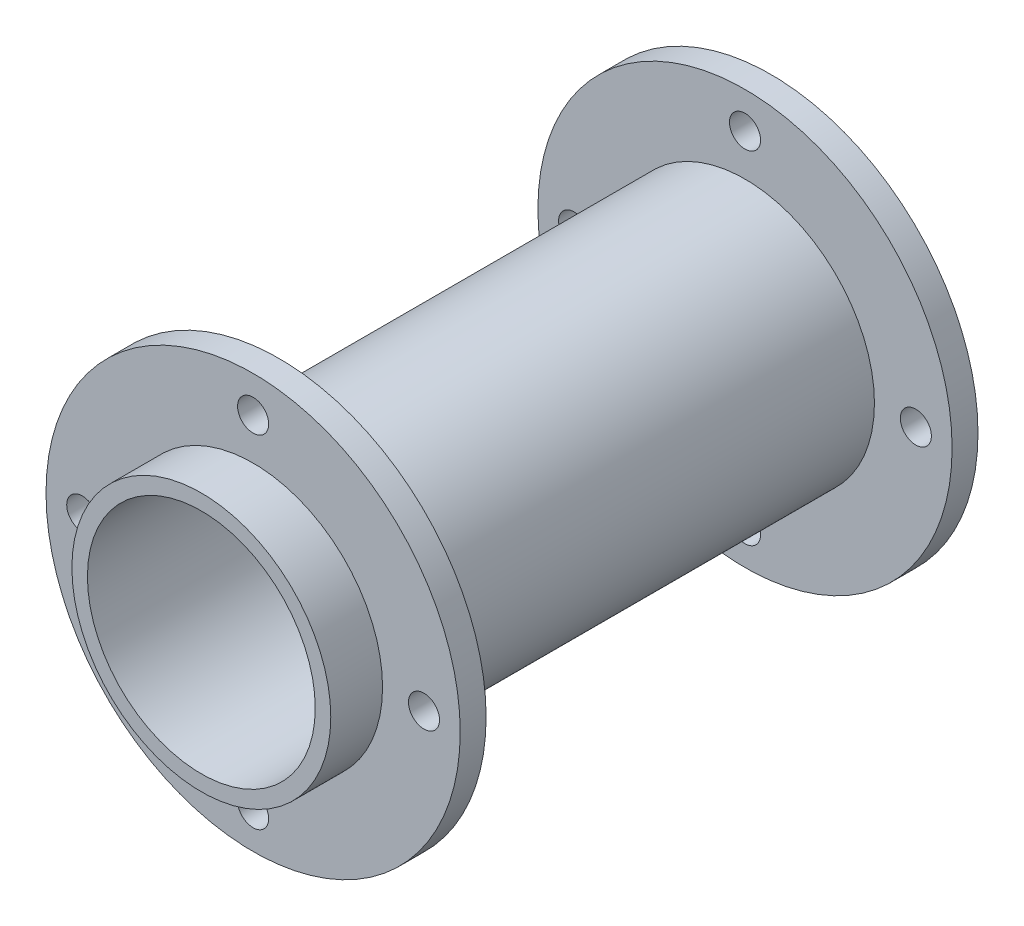
from build123d import *

# Parameters (mm, degrees)
SKETCH1_R           = 25
SKETCH1_R_2         = 22
BOSS_EXTRUDE1_DEPTH = 60
BOSS_EXTRUDE2_START = -15
SKETCH2_R           = 40
SKETCH2_R_2         = 25
SKETCH2_R_3         = 3
BOSS_EXTRUDE2_DEPTH = 5


with BuildPart() as part:
    # Sketch1 → Boss-Extrude1 (new, symmetric)
    with BuildSketch(Plane.XY):
        Circle(SKETCH1_R)
        Circle(SKETCH1_R_2, mode=Mode.SUBTRACT)
    extrude(amount=BOSS_EXTRUDE1_DEPTH, both=True)

    # Sketch2 → Boss-Extrude2 (add)
    with BuildSketch(Plane(origin=(0, 0, -60), x_dir=(-1, 0, 0), z_dir=(0, 0, -1)).offset(BOSS_EXTRUDE2_START)):
        Circle(SKETCH2_R)
        Circle(SKETCH2_R_2, mode=Mode.SUBTRACT)
        with Locations((0, 33)):
            Circle(SKETCH2_R_3, mode=Mode.SUBTRACT)
        with Locations((33, 0)):
            Circle(SKETCH2_R_3, mode=Mode.SUBTRACT)
        with Locations((0, -33)):
            Circle(SKETCH2_R_3, mode=Mode.SUBTRACT)
        with Locations((-33, 0)):
            Circle(SKETCH2_R_3, mode=Mode.SUBTRACT)
    boss_extrude2 = extrude(amount=BOSS_EXTRUDE2_DEPTH)

    # Mirror1: Boss-Extrude2 across plane
    add(boss_extrude2.mirror(Plane.XY))


solid = part.part
